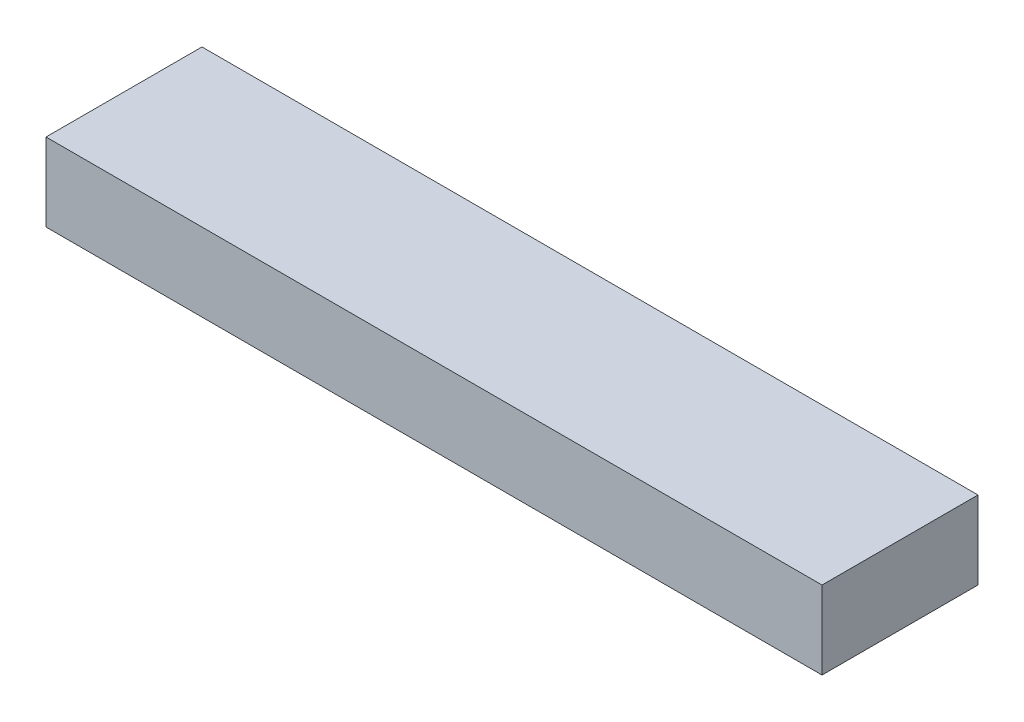
SolidWorks part; units mm, degrees
ref_plane "Front Plane" through (0, 0, 0) normal (0, 0, 1) x (1, 0, 0)
ref_plane "Top Plane" through (0, 0, 0) normal (0, 1, 0) x (1, 0, 0)
ref_plane "Right Plane" through (0, 0, 0) normal (1, 0, 0) x (0, 0, -1)
sketch "Sketch1" plane through (0, 0, 0) normal (0, 1, 0) x (1, 0, 0)
  line L1 (0, 0) -> (199, 0)
  line L2 (0, 0) -> (0, 40)
  line L3 (0, 40) -> (199, 40)
  line L4 (199, 0) -> (199, 40)
  dimension "D1" = 199
  dimension "D2" = 40
extrude "Boss-Extrude1" add sketch "Sketch1" along normal blind 20
